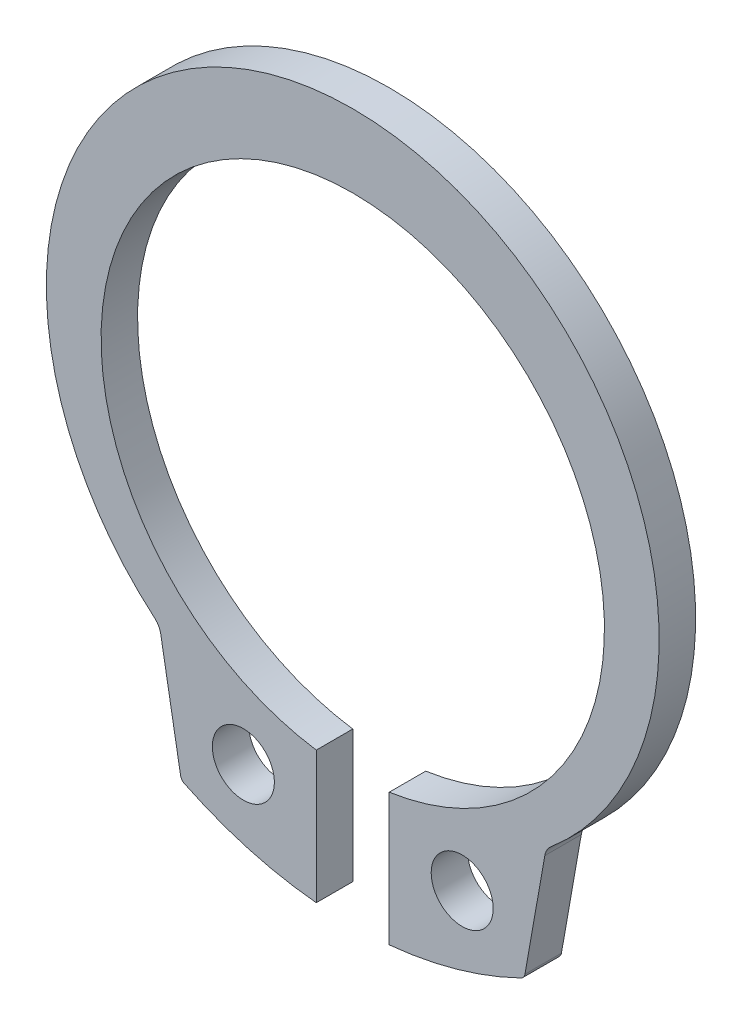
from build123d import *

# Parameters (mm, degrees)
SKETCH_1_R      = 0.85
EXTRUDE_1_DEPTH = 1


with BuildPart() as part:
    # 草图1 → 凸台-拉伸1 (new body)
    with BuildSketch(Plane.XY):
        with BuildLine():
            Line((-5.265127147, -6.69998934), (-4.720591752, -9.788203027))
            ThreePointArc((-4.720591752, -9.788203027), (-4.683411954, -9.873763838), (-4.611467681, -9.933152486))
            ThreePointArc((-4.611467681, -9.933152486), (-2.851630021, -10.605355324), (-1, -10.95227248))
            Line((-1, -10.95227248), (-1, -7.327151675))
            ThreePointArc((-1, -7.327151675), (0, 6.4), (1, -7.327151675))
            Line((1, -7.327151675), (1, -10.95227248))
            ThreePointArc((1, -10.95227248), (2.851630021, -10.605355324), (4.611467681, -9.933152486))
            ThreePointArc((4.611467681, -9.933152486), (4.683411954, -9.873763838), (4.720591752, -9.788203027))
            Line((4.720591752, -9.788203027), (5.265127147, -6.69998934))
            ThreePointArc((5.265127147, -6.69998934), (5.323845106, -6.537983114), (5.434074225, -6.405531775))
            ThreePointArc((5.434074225, -6.405531775), (0, 8.4), (-5.434074225, -6.405531775))
            ThreePointArc((-5.434074225, -6.405531775), (-5.323845106, -6.537983114), (-5.265127147, -6.69998934))
        make_face()
        with Locations(Location((3, -8.666394553, 0), (0, 0, 180))):
            Circle(SKETCH_1_R, mode=Mode.SUBTRACT)
        with Locations(Location((-3, -8.666394553, 0), (0, 0, 180))):
            Circle(SKETCH_1_R, mode=Mode.SUBTRACT)
    extrude(amount=-EXTRUDE_1_DEPTH)


solid = part.part
